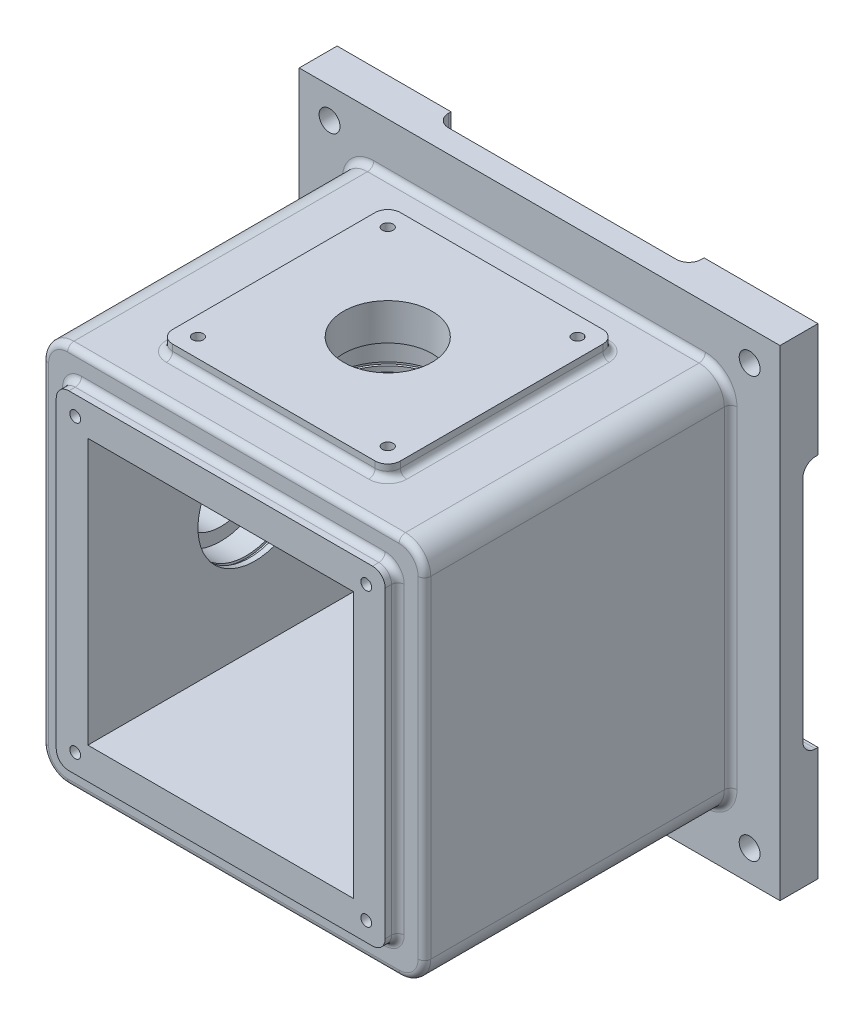
from build123d import *

# Parameters (mm, degrees)
SKETCH_1_W              = 380
SKETCH_1_H              = 380
SKETCH_1_R              = 8.25
EXTRUDE_1_DEPTH         = 30
CUT_EXTRUDE_1_DEPTH     = 426.910788781
CUT_EXTRUDE_2_DEPTH     = 426.910788781
EXTRUDE_2_DEPTH         = 242
EXTRUDE_3_DEPTH         = 10
EXTRUDE_5_DEPTH         = 10
HOLE_WIZARD_M10_1_D     = 8.5
HOLE_WIZARD_M10_1_DEPTH = 22
HOLE_WIZARD_M10_1_TIP   = 2.553657631
HOLE_WIZARD_M10_3_D     = 8.5
HOLE_WIZARD_M10_3_DEPTH = 22
HOLE_WIZARD_M10_3_TIP   = 2.553657631
SKETCH_14_W             = 210
SKETCH_14_H             = 210
CUT_EXTRUDE_3_DEPTH     = 252
SKETCH_15_R             = 90
EXTRUDE_6_DEPTH         = 20
FILLET_1_R              = 5
CUT_EXTRUDE_4_REACH     = 490.697
SKETCH_18_R             = 35
CUT_EXTRUDE_5_REACH     = 497.928
SKETCH_19_R             = 35
SKETCH_20_R             = 45
CUT_EXTRUDE_6_DEPTH     = 27
SKETCH_21_R             = 45
CUT_EXTRUDE_7_DEPTH     = 27
HOLE_WIZARD_M10_4_D     = 8.5
HOLE_WIZARD_M10_4_DEPTH = 22
HOLE_WIZARD_M10_4_TIP   = 2.553657631
FILLET_2_R              = 5
SKETCH_24_R             = 46.75
CUT_EXTRUDE_8_DEPTH     = 2.7
SKETCH_25_R             = 46.75
CUT_EXTRUDE_9_DEPTH     = 2.7


with BuildPart() as part:
    # 草图1 → 凸台-拉伸1 (new body)
    with BuildSketch(Plane.XY):
        Rectangle(SKETCH_1_W, SKETCH_1_H)
        with Locations((-166, 166)):
            Circle(SKETCH_1_R, mode=Mode.SUBTRACT)
        with Locations((166, 166)):
            Circle(SKETCH_1_R, mode=Mode.SUBTRACT)
        with Locations((166, -166)):
            Circle(SKETCH_1_R, mode=Mode.SUBTRACT)
        with Locations((-166, -166)):
            Circle(SKETCH_1_R, mode=Mode.SUBTRACT)
    extrude(amount=EXTRUDE_1_DEPTH)

    # 草图2 → 切除-拉伸1 (cut, through all)
    with BuildSketch(Plane.XZ.offset(190)):
        with BuildLine():
            Line((-100, 0), (-100, 2))
            ThreePointArc((-100, 2), (-97.071067812, 9.071067812), (-90, 12))
            Line((-90, 12), (90, 12))
            ThreePointArc((90, 12), (97.071067812, 9.071067812), (100, 2))
            Line((100, 2), (100, 0))
            Line((100, 0), (-100, 0))
        make_face()
    extrude(amount=-CUT_EXTRUDE_1_DEPTH, mode=Mode.SUBTRACT)

    # 草图3 → 切除-拉伸2 (cut, through all)
    with BuildSketch(Plane(origin=(190, 0, 0), x_dir=(0, 0, -1), z_dir=(1, 0, 0))):
        with BuildLine():
            Line((0, -100), (-2, -100))
            ThreePointArc((-2, -100), (-9.071067812, -97.071067812), (-12, -90))
            Line((-12, -90), (-12, 90))
            ThreePointArc((-12, 90), (-9.071067812, 97.071067812), (-2, 100))
            Line((-2, 100), (0, 100))
            Line((0, 100), (0, -100))
        make_face()
    extrude(amount=-CUT_EXTRUDE_2_DEPTH, mode=Mode.SUBTRACT)

    # 草图4 → 凸台-拉伸2 (add)
    with BuildSketch(Plane.XY.offset(30)):
        with BuildLine():
            Line((-131, 151), (131, 151))
            ThreePointArc((131, 151), (145.142135624, 145.142135624), (151, 131))
            Line((151, 131), (151, -131))
            ThreePointArc((151, -131), (145.142135624, -145.142135624), (131, -151))
            Line((131, -151), (-131, -151))
            ThreePointArc((-131, -151), (-145.142135624, -145.142135624), (-151, -131))
            Line((-151, -131), (-151, 131))
            ThreePointArc((-151, 131), (-145.142135624, 145.142135624), (-131, 151))
        make_face()
    extrude(amount=EXTRUDE_2_DEPTH)

    # 草图5 → 凸台-拉伸3 (add)
    with BuildSketch(Plane(origin=(0, 151, 0), x_dir=(1, 0, 0), z_dir=(0, 1, 0))):
        with BuildLine():
            Line((80, -240), (-80, -240))
            ThreePointArc((-80, -240), (-87.071067812, -237.071067812), (-90, -230))
            Line((-90, -230), (-90, -70))
            ThreePointArc((-90, -70), (-87.071067812, -62.928932188), (-80, -60))
            Line((-80, -60), (80, -60))
            ThreePointArc((80, -60), (87.071067812, -62.928932188), (90, -70))
            Line((90, -70), (90, -230))
            ThreePointArc((90, -230), (87.071067812, -237.071067812), (80, -240))
        make_face()
    extrude(amount=EXTRUDE_3_DEPTH)

    # 草图7 → 凸台-拉伸5 (add)
    with BuildSketch(Plane.XY.offset(272)):
        with BuildLine():
            Line((-120, -130), (120, -130))
            ThreePointArc((120, -130), (127.071067812, -127.071067812), (130, -120))
            Line((130, -120), (130, 120))
            ThreePointArc((130, 120), (127.071067812, 127.071067812), (120, 130))
            Line((120, 130), (-120, 130))
            ThreePointArc((-120, 130), (-127.071067812, 127.071067812), (-130, 120))
            Line((-130, 120), (-130, -120))
            ThreePointArc((-130, -120), (-127.071067812, -127.071067812), (-120, -130))
        make_face()
    extrude(amount=EXTRUDE_5_DEPTH)

    # M10 螺纹孔1
    with Locations(Plane(origin=(75, 161, 225), x_dir=(0, 0, 1), z_dir=(0, 1, 0))):
        with Locations((0, 0), (0, -150), (-150, -150), (-150, 0)):
            Hole(HOLE_WIZARD_M10_1_D / 2, depth=HOLE_WIZARD_M10_1_DEPTH)
            with Locations((0, 0, -(HOLE_WIZARD_M10_1_DEPTH + HOLE_WIZARD_M10_1_TIP / 2))):  # 118° drill point
                Cone(0, HOLE_WIZARD_M10_1_D / 2, HOLE_WIZARD_M10_1_TIP, mode=Mode.SUBTRACT)

    # M10 螺纹孔3
    with Locations(Plane(origin=(115, -115, 282), x_dir=(1, 0, 0), z_dir=(0, 0, 1))):
        with Locations((0, 0), (0, 230), (-230, 230), (-230, 0)):
            Hole(HOLE_WIZARD_M10_3_D / 2, depth=HOLE_WIZARD_M10_3_DEPTH)
            with Locations((0, 0, -(HOLE_WIZARD_M10_3_DEPTH + HOLE_WIZARD_M10_3_TIP / 2))):  # 118° drill point
                Cone(0, HOLE_WIZARD_M10_3_D / 2, HOLE_WIZARD_M10_3_TIP, mode=Mode.SUBTRACT)

    # 草图14 → 切除-拉伸3 (cut)
    with BuildSketch(Plane.XY.offset(282)):
        Rectangle(SKETCH_14_W, SKETCH_14_H)
    extrude(amount=-CUT_EXTRUDE_3_DEPTH, mode=Mode.SUBTRACT)

    # 草图15 → 凸台-拉伸6 (add)
    with BuildSketch(Plane.ZY.offset(151)):
        with Locations(Location((150, 0, 0), (0, 0, 90))):
            Circle(SKETCH_15_R)
    extrude(amount=EXTRUDE_6_DEPTH)

    # 圆角1
    fillet_1_edges = [part.edges().sort_by_distance(p)[0] for p in [
        (-145.142135624, -145.142135624, 30),
        (0, -151, 30),
        (145.142135624, -145.142135624, 30),
        (151, 0, 30),
        (145.142135624, 145.142135624, 30),
        (0, 151, 30),
        (-145.142135624, 145.142135624, 30),
        (-151, 0, 30),
        (-145.142135624, -145.142135624, 272),
        (0, -151, 272),
        (145.142135624, -145.142135624, 272),
        (151, 0, 272),
        (145.142135624, 145.142135624, 272),
        (0, 151, 272),
        (-145.142135624, 145.142135624, 272),
        (-151, 0, 272),
        (87.071067812, 151, 62.928932188),
        (0, 151, 60),
        (-87.071067812, 151, 62.928932188),
        (-90, 151, 150),
        (-87.071067812, 151, 237.071067812),
        (0, 151, 240),
        (87.071067812, 151, 237.071067812),
        (90, 151, 150),
        (127.071067812, -127.071067812, 272),
        (130, 0, 272),
        (127.071067812, 127.071067812, 272),
        (0, 130, 272),
        (-127.071067812, 127.071067812, 272),
        (-130, 0, 272),
        (-127.071067812, -127.071067812, 272),
        (0, -130, 272),
    ]]
    fillet(fillet_1_edges, radius=FILLET_1_R)

    # 草图18 → 切除-拉伸4 (cut, up to next)
    with BuildSketch(Plane(origin=(0, 161, 0), x_dir=(1, 0, 0), z_dir=(0, 1, 0)), mode=Mode.PRIVATE) as cut_extrude_4_sk1:
        with Locations(Location((0, -150, 0), (0, 0, 270))):
            Circle(SKETCH_18_R)
    cut_extrude_4_tool1 = extrude(cut_extrude_4_sk1.sketch, amount=-CUT_EXTRUDE_4_REACH, mode=Mode.PRIVATE) & part.part
    add(cut_extrude_4_tool1.solids().sort_by_distance((0, 161, 150))[0], mode=Mode.SUBTRACT)

    # 草图19 → 切除-拉伸5 (cut, up to next)
    with BuildSketch(Plane.ZY.offset(171), mode=Mode.PRIVATE) as cut_extrude_5_sk1:
        with Locations(Location((150, 0, 0), (0, 0, 270))):
            Circle(SKETCH_19_R)
    cut_extrude_5_tool1 = extrude(cut_extrude_5_sk1.sketch, amount=-CUT_EXTRUDE_5_REACH, mode=Mode.PRIVATE) & part.part
    add(cut_extrude_5_tool1.solids().sort_by_distance((-171, 0, 150))[0], mode=Mode.SUBTRACT)

    # 草图20 → 切除-拉伸6 (cut)
    with BuildSketch(Plane.XZ.offset(-105)):
        with Locations(Location((0, 150, 0), (0, 0, 270))):
            Circle(SKETCH_20_R)
    extrude(amount=-CUT_EXTRUDE_6_DEPTH, mode=Mode.SUBTRACT)

    # 草图21 → 切除-拉伸7 (cut)
    with BuildSketch(Plane(origin=(-105, 0, 0), x_dir=(0, 0, -1), z_dir=(1, 0, 0))):
        with Locations((-150, 0)):
            Circle(SKETCH_21_R)
    extrude(amount=-CUT_EXTRUDE_7_DEPTH, mode=Mode.SUBTRACT)

    # M10 螺纹孔4
    with Locations(Plane(origin=(-171, 0, 225), x_dir=(0, -1, 0), z_dir=(-1, 0, 0))):
        with Locations((0, 0), (64.951905284, -37.5), (64.951905284, -112.5), (0, -150), (-64.951905284, -112.5), (-64.951905284, -37.5)):
            Hole(HOLE_WIZARD_M10_4_D / 2, depth=HOLE_WIZARD_M10_4_DEPTH)
            with Locations((0, 0, -(HOLE_WIZARD_M10_4_DEPTH + HOLE_WIZARD_M10_4_TIP / 2))):  # 118° drill point
                Cone(0, HOLE_WIZARD_M10_4_D / 2, HOLE_WIZARD_M10_4_TIP, mode=Mode.SUBTRACT)

    # 圆角2
    fillet_2_edges = [part.edges().sort_by_distance(p)[0] for p in [
        (-151, -90, 150),
    ]]
    fillet(fillet_2_edges, radius=FILLET_2_R)

    # 草图24 → 切除-拉伸8 (cut)
    with BuildSketch(Plane(origin=(-112, 0, 0), x_dir=(0, 0, -1), z_dir=(1, 0, 0))):
        with Locations(Location((-150, 0, 0), (0, 0, 180))):
            Circle(SKETCH_24_R)
    extrude(amount=CUT_EXTRUDE_8_DEPTH, mode=Mode.SUBTRACT)

    # 草图25 → 切除-拉伸9 (cut)
    with BuildSketch(Plane(origin=(0, 112, 0), x_dir=(-1, 0, 0), z_dir=(0, -1, 0))):
        with Locations(Location((0, -150, 0), (0, 0, 270))):
            Circle(SKETCH_25_R)
    extrude(amount=CUT_EXTRUDE_9_DEPTH, mode=Mode.SUBTRACT)


solid = part.part
